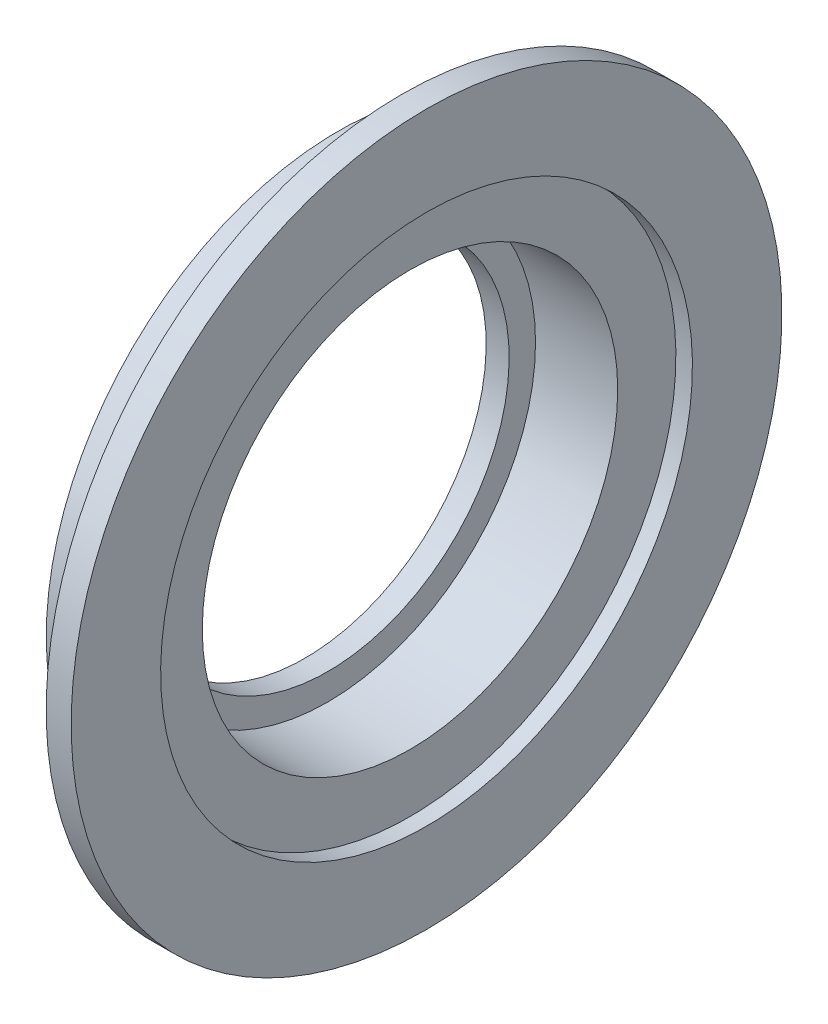
SolidWorks part; units mm, degrees
ref_plane "Front Plane" through (0, 0, 0) normal (0, 0, 1) x (1, 0, 0)
ref_plane "Top Plane" through (0, 0, 0) normal (0, 1, 0) x (1, 0, 0)
ref_plane "Right Plane" through (0, 0, 0) normal (1, 0, 0) x (0, 0, -1)
sketch "Sketch1" plane through (0, 0, 0) normal (0, 0, 1) x (1, 0, 0)
  line L0 (0, 0) -> (-17.3889, 0) construction
  line L1 (107, 42) -> (107, 35)
  line L2 (107, 33.7491) -> (107, 42) construction
  line L3 (107, 114) -> (107, 33.7491) construction
  line L4 (107, -35) -> (107, 35) construction
  line L5 (107, 35) -> (104.5085, 35)
  line L6 (104.5085, 35) -> (104.5085, 27.05)
  line L7 (104.5085, 27.05) -> (95.5713, 27.05)
  line L8 (95.5713, 27.05) -> (95.5713, 21.4326)
  line L9 (95.5713, 21.4326) -> (98.2863, 21.4326)
  line L10 (98.2863, 21.4326) -> (98.2863, 24.55)
  line L11 (98.2863, 24.55) -> (108, 24.55)
  line L12 (109.9542, 31.426) -> (109.9542, 42)
  line L13 (109.9542, 42) -> (107, 42)
  line L14 (109.9542, 31.426) -> (108, 31.426)
  line L15 (108, 114) -> (108, 0) construction
  line L16 (108, 31.426) -> (108, 24.55)
revolve "Revolve1" add sketch "Sketch1" angle 360 about L0
sketch "Sketch2" plane through (104.5085, 0, 0) normal (-1, 0, 0) x (0, 0, 1)
  circle A0 centre (0, 0) radius 29.5
  circle A1 centre (0, 0) radius 30.5
  circle A2 centre (0, 0) radius 33.5
  circle A3 centre (0, 0) radius 34.5
  dimension "D1" = 1
  dimension "D2" = 3
  dimension "D3" = 1
extrude "Boss-Extrude1" add sketch "Sketch2" along normal blind 5 contours A1 A0 | A3 A2
